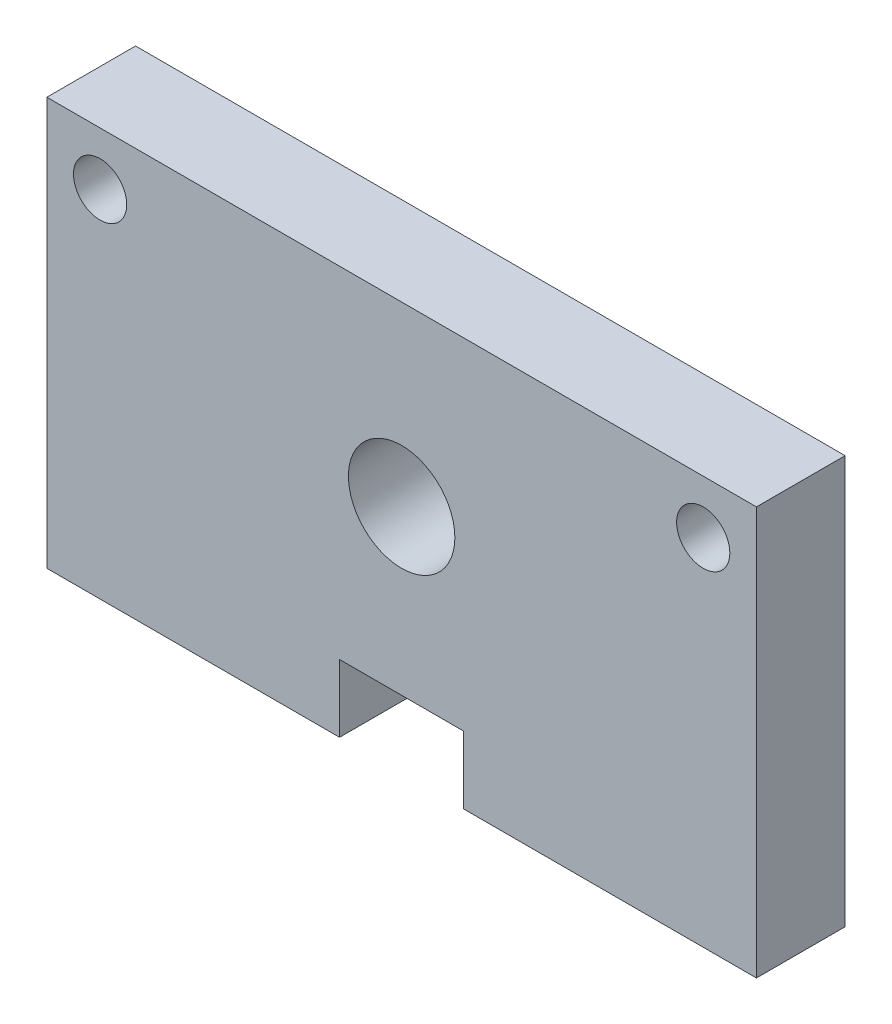
from build123d import *

# Parameters (mm, degrees)
SKETCH1_R           = 3
SKETCH1_R_2         = 1.5
BOSS_EXTRUDE1_DEPTH = 5


with BuildPart() as part:
    # Sketch1 → Boss-Extrude1 (new body)
    with BuildSketch(Plane.XY):
        Polygon((-20, -10), (-20, 10), (20, 10), (20, -10), (20, -13), (3.5, -13), (3.5, -9.2), (-3.5, -9.2), (-3.5, -13), (-20, -13), align=None)
        Circle(SKETCH1_R, mode=Mode.SUBTRACT)
        with Locations((-17, 7)):
            Circle(SKETCH1_R_2, mode=Mode.SUBTRACT)
        with Locations((17, 7)):
            Circle(SKETCH1_R_2, mode=Mode.SUBTRACT)
    extrude(amount=BOSS_EXTRUDE1_DEPTH)


solid = part.part
